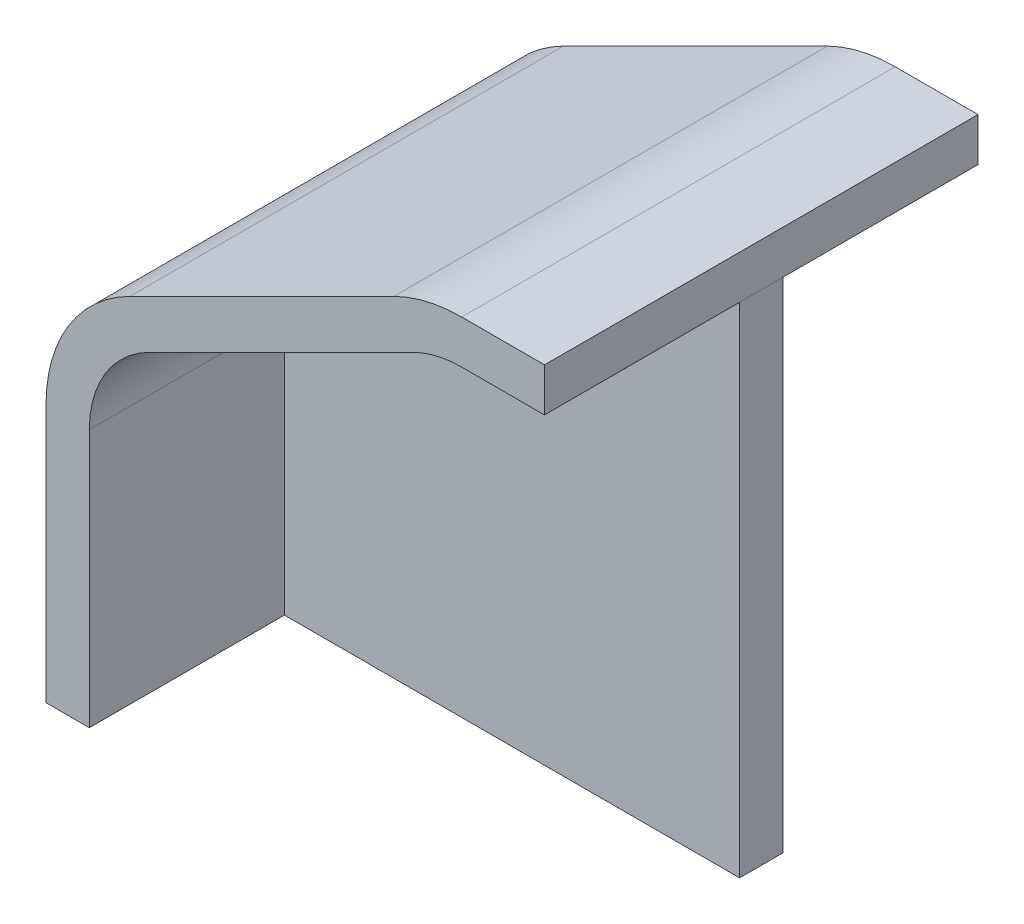
from build123d import *

# Parameters (mm, degrees)
EXTRUDE_1_DEPTH = 20
EXTRUDE_2_DEPTH = 100


with BuildPart() as part:
    # 草图1 → 凸台-拉伸1 (new body)
    with BuildSketch(Plane.XY):
        with BuildLine():
            Line((0, 0), (210, 0))
            Line((210, 0), (210, 230))
            Line((210, 230), (171.803398875, 230))
            ThreePointArc((171.803398875, 230), (160.315752848, 228.662449473), (149.4427191, 224.72135955))
            Line((149.4427191, 224.72135955), (27.639320225, 163.819660113))
            ThreePointArc((27.639320225, 163.819660113), (7.467459582, 145.384856168), (0, 119.098300563))
            Line((0, 119.098300563), (0, 0))
        make_face()
    extrude(amount=EXTRUDE_1_DEPTH)


with BuildPart() as body_2:
    # 草图2 → 凸台-拉伸2 (new, symmetric)
    with BuildSketch(Plane.XY.offset(10)):
        with BuildLine():
            Line((210, 250), (171.803398875, 250))
            ThreePointArc((171.803398875, 250), (155.720694437, 248.127429263), (140.49844719, 242.60990337))
            Line((140.49844719, 242.60990337), (18.695048315, 181.708203932))
            ThreePointArc((18.695048315, 181.708203932), (-9.545556585, 155.899478411), (-20, 119.098300563))
            Line((-20, 119.098300563), (-20, 0))
            Line((-20, 0), (0, 0))
            Line((0, 0), (0, 119.098300563))
            ThreePointArc((0, 119.098300563), (7.467459582, 145.384856168), (27.639320225, 163.819660113))
            Line((27.639320225, 163.819660113), (149.4427191, 224.72135955))
            ThreePointArc((149.4427191, 224.72135955), (160.315752848, 228.662449473), (171.803398875, 230))
            Line((171.803398875, 230), (210, 230))
            Line((210, 230), (210, 250))
        make_face()
    extrude(amount=EXTRUDE_2_DEPTH, both=True)


solid = Compound([part.part, body_2.part])
